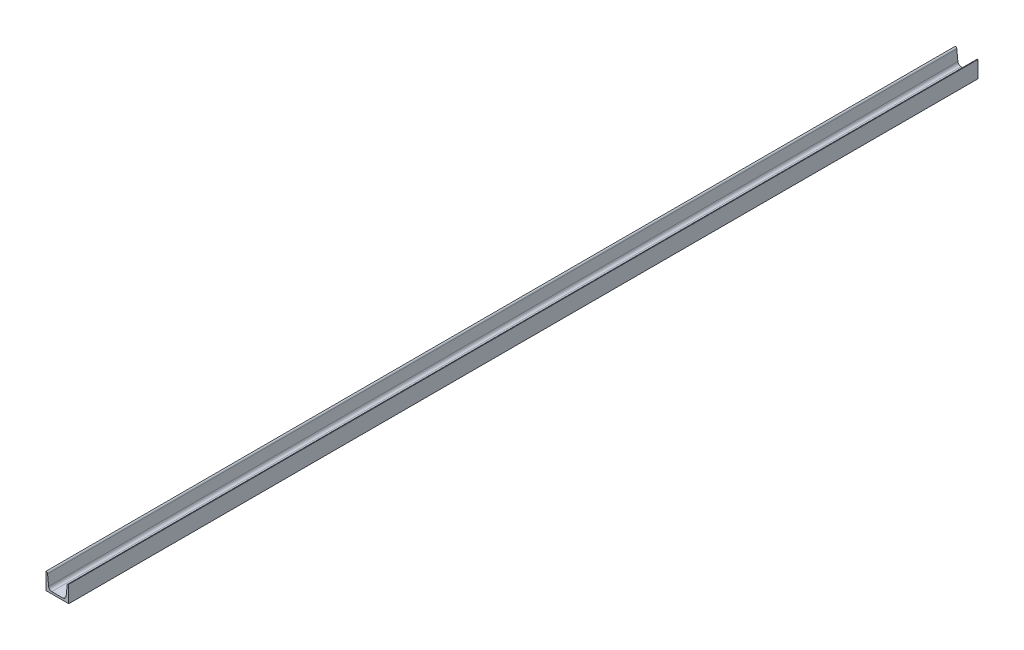
from build123d import *

# Parameters (mm, degrees)
EXTRUDE1_DEPTH = 1000


with BuildPart() as part:
    # Sketch1 → Extrude1 (new, symmetric)
    with BuildSketch(Plane.XY):
        with BuildLine():
            Line((-25, 0), (25, 0))
            Line((25, 0), (25, 37))
            ThreePointArc((25, 37), (22.671841203, 36.084021126), (21.549999087, 33.847771823))
            Line((21.549999087, 33.847771823), (19.250000913, 10.804761752))
            ThreePointArc((19.250000913, 10.804761752), (16.982128941, 6.310266493), (12.284611923, 4.5))
            Line((12.284611923, 4.5), (-12.284611923, 4.5))
            ThreePointArc((-12.284611923, 4.5), (-16.982128941, 6.310266493), (-19.250000913, 10.804761752))
            Line((-19.250000913, 10.804761752), (-21.549999087, 33.847771823))
            ThreePointArc((-21.549999087, 33.847771823), (-22.671841203, 36.084021126), (-25, 37))
            Line((-25, 37), (-25, 0))
        make_face()
    extrude(amount=EXTRUDE1_DEPTH, both=True)


solid = part.part
